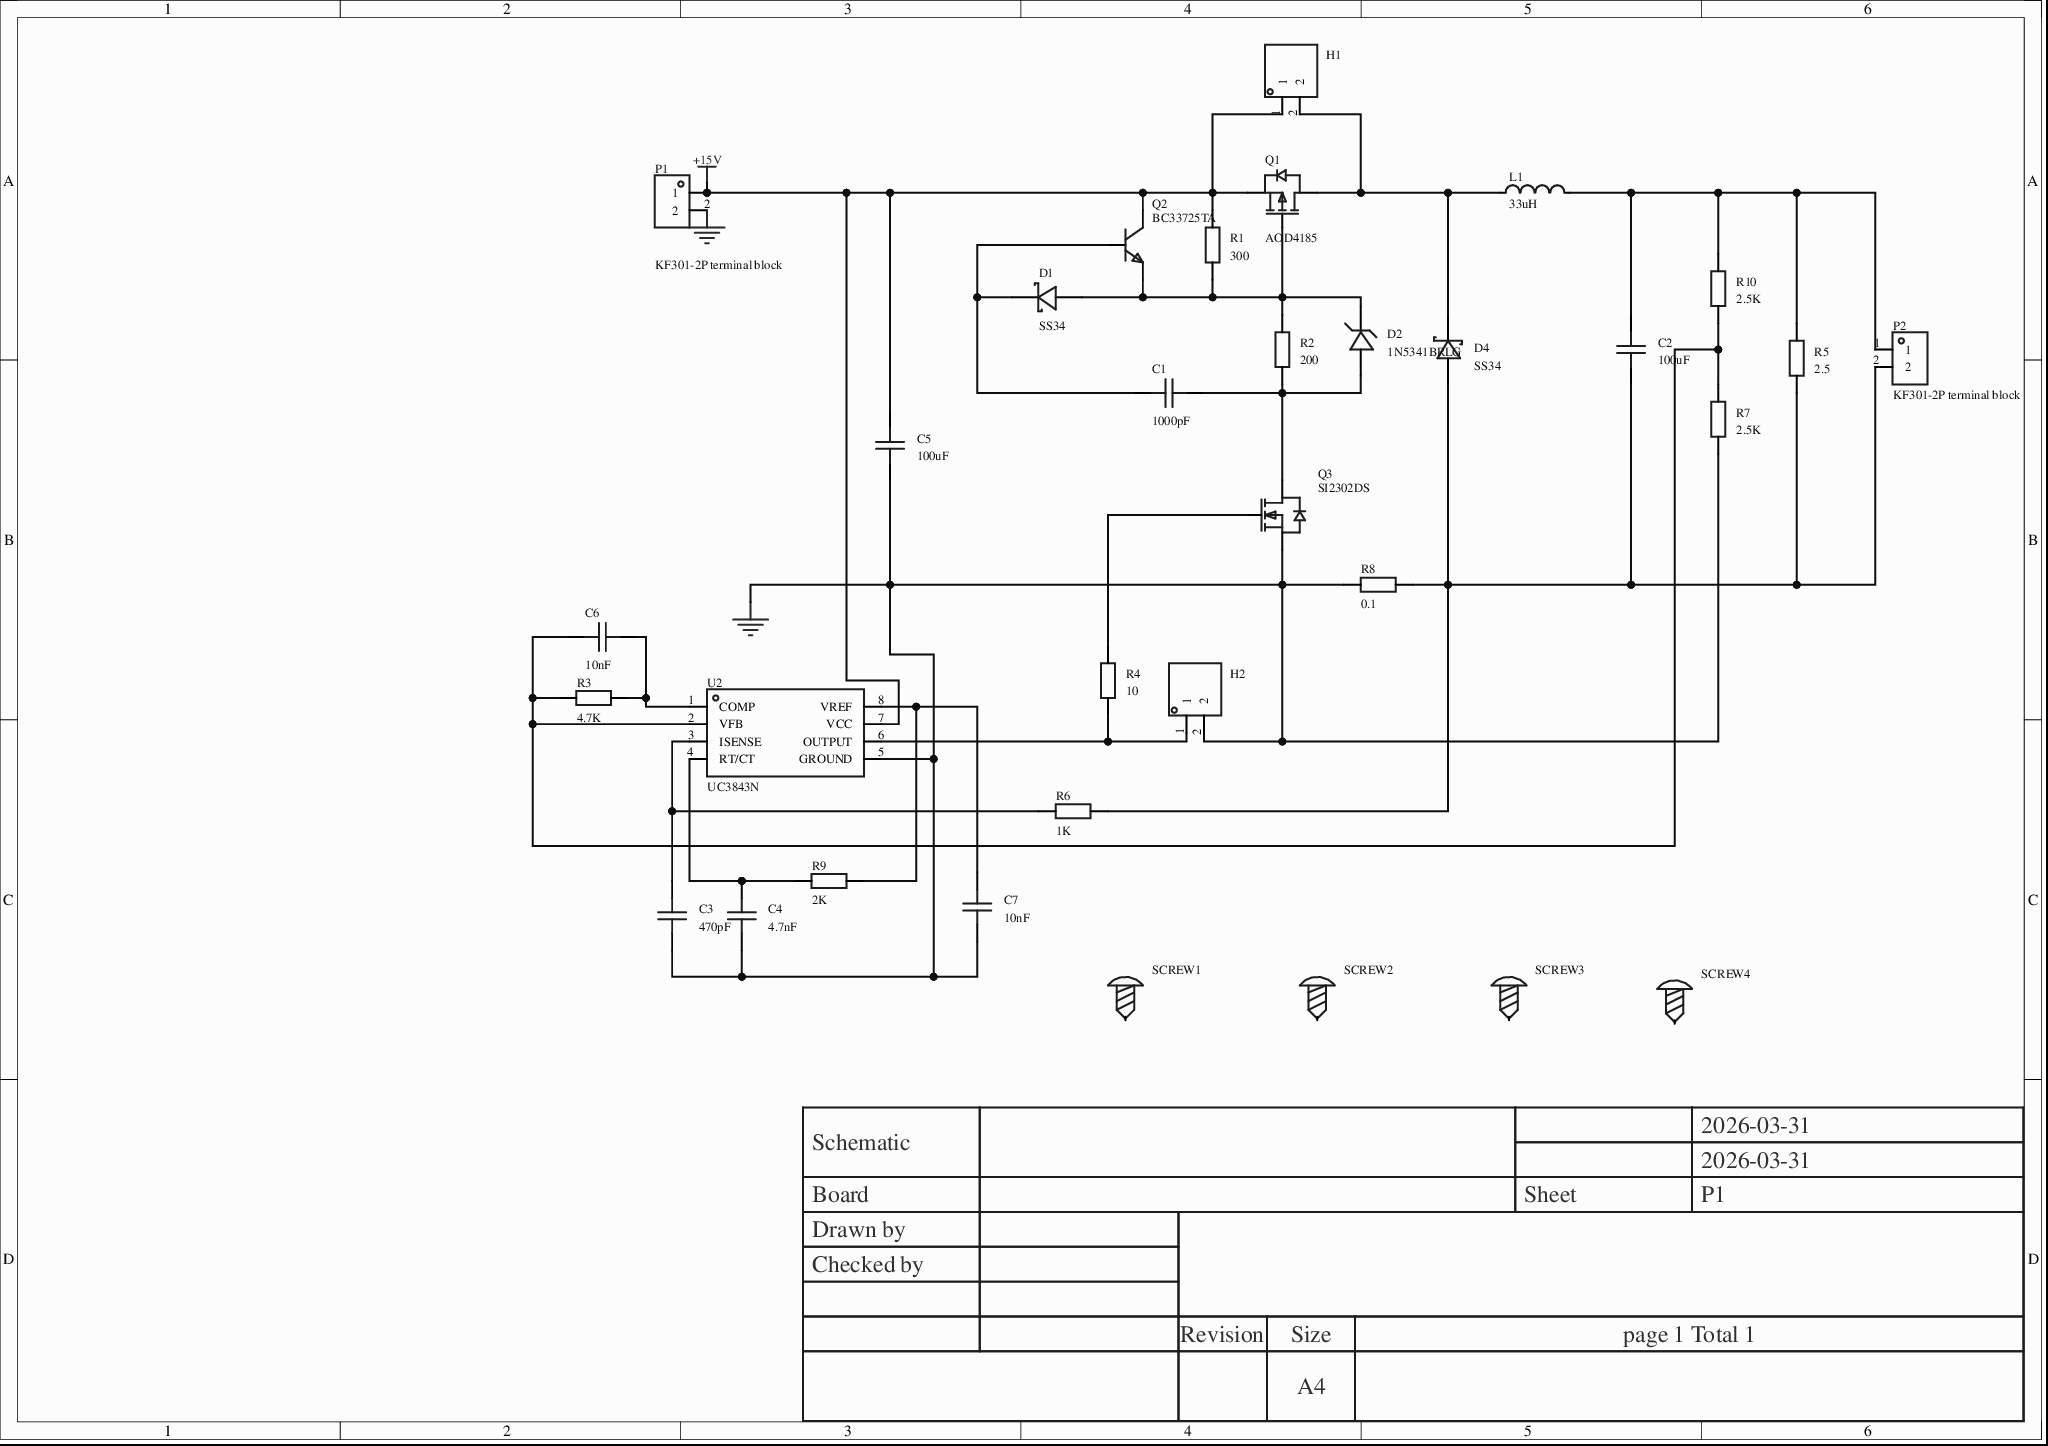
[diagram p0: MISC50807-3.schdoc]
# Altium project MISC50807-2.PrjPcb
1 sheet, 33 parts. Net scope: global (net labels, ports and power ports of the same name join across sheets).
Board file: MISC50807.pcbdoc

## Sheet MISC50807-3.schdoc
size 297 x 209 mm; Version: V1.0; @Project Name: MISC50807; @Update Date: 2026-04-21; @Create Date: 2026-04-21; @Board Name: MISC50807; @Create Time: 11:05:11; @Page Count: 1; @Page No: 1; @Schematic Name: MISC50807; @Update Time: 11:05:11; Size: A4

### Parts
C1  1000pF  [CAP-TH_L5.0-W2.5-P5.00-D1.0]
C2  100uF  [CAP-TH_BD8.0-P3.50-D0.6-FD_1]
C3  470pF  [CAP-TH_L5.0-W2.5-P5.00-D1.0]
C4  4.7nF  [CAP-TH_L5.0-W2.5-P5.00-D1.0]
C5  100uF  [CAP-TH_BD8.0-P3.50-D0.6-FD_1]
C6  10nF  [CAP-TH_L5.0-W2.5-P5.00-D1.0]
C7  10nF  [C0603]
D1  SS34  [DO-15_BD3.1-L6.7-P10.70-D0.8-RD]
D2  1N5341BRLG  [DO-15_BD3.1-L6.7-P10.70-D0.8-RD]
D4  SS34  [DO-15_BD3.1-L6.7-P10.70-D0.8-RD]
H1  (no value)  [HDR-TH_2P-P2.54-V-M-1]
H2  (no value)  [HDR-TH_2P-P2.54-V-M-1]
L1  33uH  [IND-TH_BD7.8-P5.00-D0.7]
P1  KF301-2P terminal block  [CONN-TH_XY301V-A-5.0-2P]
P2  KF301-2P terminal block  [CONN-TH_XY301V-A-5.0-2P]
Q1  AOD4185  [SOT-23-3_L2.9-W1.3-P1.90-LS2.4-L]
Q2  BC33725TA  [TO-92-3_L4.9-W3.7-P2.54-L]
Q3  SI2302DS  [SOT-23-3_L2.9-W1.3-P1.90-LS2.4-L]
R1  300  [Res_1/4W]
R2  200  [Res_1/4W]
R3  4.7K  [Res_1/4W]
R4  10  [Res_1/4W]
R5  2.5  [Res_1/4W]
R6  1K  [Res_1/4W]
R7  2.5K  [Res_1/4W]
R8  0.1  [Res_1/4W]
R9  2K  [Res_1/4W]
R10  2.5K  [Res_1/4W]
SCREW1  (no value)  [M3螺丝]
SCREW2  (no value)  [M3螺丝]
SCREW3  (no value)  [M3螺丝]
SCREW4  (no value)  [M3螺丝]
U2  UC3843N  [SOP-8_L5.1-W3.9-P1.27-LS6.0-BL]

### Nets
+15V: C5.2 H1.1 P1.1 Q1.3(S) Q2.1(C) R1.1 U2.7(VCC)
GND: C3.1 C4.1 C5.1 C7.1 H2.2 P1.2 Q3.2(S) R7.1 R8.1 U2.5(GROUND)
NetC1_1: C1.1 D1.1(C) Q2.2(B)
NetC1_2: C1.2 D2.2(A) Q3.3(D) R2.2
NetC2_1: C2.1 D4.2(A) P2.2 R5.1 R6.2 R8.2
NetC2_2: C2.2 L1.2 P2.1 R5.2 R10.2
NetC3_2: C3.2 R6.1 U2.3(ISENSE)
NetC4_2: C4.2 R9.1 U2.4(RT/CT)
NetC6_1: C6.1 R3.1 R7.2 R10.1 U2.2(VFB)
NetC6_2: C6.2 R3.2 U2.1(COMP)
NetC7_2: C7.2 R9.2 U2.8(VREF)
NetD1_2: D1.2(A) D2.1(C) Q1.1(G) Q2.3(E) R1.2 R2.1
NetD4_1: D4.1(C) H1.2 L1.1 Q1.2(D)
NetH2_1: H2.1 R4.2 U2.6(OUTPUT)
NetQ3_1: Q3.1(G) R4.1

Not connected (* = marked no-connect by the designer): SCREW1 1; SCREW2 1; SCREW3 1; SCREW4 1

### Notes on the sheet
- 2026-03-31
- Schematic
- Board
- Sheet
- P1
- Drawn by
- Checked by
- Revision
- Size
- A4
- page 1 Total 1

### Library data of the parts
C1-C4 = CAP_0603: Symbol: Capacitance; ConvertToPcb: yes; ModelId: ac125912035d415993ca9572d50418b10819f05c4eef4c71ace90d822a990e87; ModelName: C0603_L1.6-W0.8-H0.8; ModelTransform: 62.992,31.496,0,0,0,0,0,0,0; Device: CAP_0603; AddInBom: yes; Supplier Footprint: 0603
  C1: Value: 1000pF; FootprintName: CAP-TH_L5.0-W2.5-P5.00-D1.0
  C2: Value: 100uF; FootprintName: CAP-TH_BD8.0-P3.50-D0.6-FD_1
  C3: Value: 470pF; FootprintName: CAP-TH_L5.0-W2.5-P5.00-D1.0
  C4: Value: 4.7nF; FootprintName: CAP-TH_L5.0-W2.5-P5.00-D1.0
C5 C6 = CAP_0603: Symbol: Capacitance; 3D Model: ac125912035d415993ca9572d50418b10819f05c4eef4c71ace90d822a990e87; 3D Model Transform: 62.992,31.496,0,0,0,0,0,0,0; ConvertToPcb: yes; ModelName: C0603_L1.6-W0.8-H0.8; Device: CAP_0603; Supplier Footprint: 0603; AddInBom: yes
  C5: Value: 100uF; FootprintName: CAP-TH_BD8.0-P3.50-D0.6-FD_1
  C6: Value: 10nF; FootprintName: CAP-TH_L5.0-W2.5-P5.00-D1.0
C7 = CAP_0603: Symbol: CapAcitance; ConvertToPcb: yes; ModelId: ac125912035d415993ca9572d50418b10819f05c4eef4c71ace90d822a990e87; ModelName: C0603_L1.6-W0.8-H0.8; ModelTransform: 62.992,31.496,0,0,0,0,0,0,0; Device: CAP_0603; Value: 10nF; AddInBom: yes; Supplier Footprint: 0603; FootprintName: C0603
D1 D4 = SS34_C154551: Forward voltage (Vf): 500mV@3A; DC reverse voltage (Vr): 40V; Rectified current: 3A;; Manufacturer: onsemi(安森美); AddInBom: yes; Reverse Leakage Current (Ir): 500uA@40V; Operating Junction Temperature Range: -55℃~+150℃; Non-Repetitive Peak Forward Surge Current: 100A; ModelId: 181deed3e51b4528a83dd624c23bafda0819f05c4eef4c71ace90d822a990e87; ModelName: SMC_L6.9-W5.9-LS7.9-RD; ModelTransform: 314.96,236.22,0,0,0,0,0,0,0; Device: SS34_C154551; Symbol: SS34_C154551; FootprintName: DO-15_BD3.1-L6.7-P10.70-D0.8-RD; LCSC Part Name: 电压:40V 电流:3A; SupplierPart: C154551; ManufacturerPart: SS34; Supplier Footprint: SMC(DO-214AB); JLCPCB Part Class: Extended Part; Datasheet: https://example.com/datasheet/SS34/165893.html; Supplier: LCSC; ConvertToPcb: yes; Voltage - Forward(Vf@If): 500mV@3A; Voltage - DC Reverse(Vr): 40V; Current - Rectified: 3A
D2 = 1N5341BRLG: Diode configuration: standalone; Zener voltage (nominal): 6.2V; Zener voltage (range): 5.89V~6.51V; Tolerance: ±5%; Power: 5W; Reverse current (Ir): 1uA@3V; Impedance (Zzt): 1Ω;; Manufacturer: onsemi(安森美); AddInBom: yes; ModelId: ac7174ae5660404daaf53aba56e542fa0819f05c4eef4c71ace90d822a990e87; ModelName: DO-27_BD3.5-L8.6-P12.60-D1.3-RD; ModelTransform: 551.18,137.73354,0,0,0,0,0,0,-196.85; Device: 1N5341BRLG; Symbol: 1N5341BRLG; FootprintName: DO-15_BD3.1-L6.7-P10.70-D0.8-RD; LCSC Part Name: 6.2V ±5% 5W; SupplierPart: C9707; ManufacturerPart: 1N5341BRLG; Supplier Footprint: AXIAL LEAD; JLCPCB Part Class: Extended Part; Datasheet: https://example.com/upload/public/pdf/source/20121103/1457706546069.pdf; Supplier: LCSC; ConvertToPcb: yes; Diode Configuration: Standalone; Zener Voltage (Nom): 6.2V; Zener Voltage (Range): 5.89V~6.51V; Power Dissipation: 5W; Reverse Leakage Current (Ir): 1uA@3V; Zener Impedance (Zzt): 1Ω
H1 H2 = HDR-M_2.54_1x2P: Symbol: 210S-1*2P L=11.6MMGold-plated black; ConvertToPcb: yes; ModelId: 79b2e9f2d70a4d68a1b7098f27c6d4c50819f05c4eef4c71ace90d822a990e87; ModelName: HDR-M-2.54_1x2; ModelTransform: 200,100,0,0,0,0,0,0,-118.11; Device: HDR-M_2.54_1x2P; FootprintName: HDR-TH_2P-P2.54-V-M-1; AddInBom: yes; SupplierPart: C124375; Supplier Footprint: 插件
L1 = L_0603: Symbol: SDFL1608S100KTF; AddInBom: yes; ModelId: 2bc5ec593d464d6ba9807aec0b5673c20819f05c4eef4c71ace90d822a990e87; ModelName: L0603_L1.6-W0.8-H0.5_BEAD; ModelTransform: 62.992,31.496,0,180,0,0,0.094,0.629,0; Device: L_0603; Value: 33uH; FootprintName: IND-TH_BD7.8-P5.00-D0.7; Supplier Footprint: L0603; ConvertToPcb: yes
P1 P2 = KF301-2P接线端子: AddInBom: yes; ModelId: ef7ead88b0f2448d904975b26718870f0819f05c4eef4c71ace90d822a990e87; ModelTransform: 417.322,299.212,0,0,0,0,11.811,-7.835,-157.48; Device: KF301-2P terminal block; Symbol: KF301-2P terminal block; FootprintName: CONN-TH_XY301V-A-5.0-2P; LCSC Part Name: KF301-2P接线端子; SupplierPart: C9900016950; ManufacturerPart: KF301-2P接线端子; Supplier Footprint: CK301-2P; JLCPCB Part Class: Extended Part; Supplier: LCSC; ConvertToPcb: yes; ModelName: CONN-TH_XY301V-A-5.0-2P
Q1 = AOD4185_C400894: Type: 1 P-channel; Drain-source voltage (Vdss): 40V; Continuous drain current (Id): 40A; On-resistance (RDS(on)@Vgs,Id): 20mΩ@4.5V,15A; Power (Pd): 62.5W; Threshold voltage (Vgs(th)@Id): 1.7V@250uA;; Manufacturer: AOS; AddInBom: yes; Total Gate Charge (Qg@Vgs): 42nC@10V; Input Capacitance (Ciss@Vds): 2.55nF@20V; Reverse Transfer Capacitance (Crss@Vds): 190pF@20V; ModelId: dee852f3c6b348a2b9d5be5dd32440810819f05c4eef4c71ace90d822a990e87; ModelName: TO-252-3_L6.6-W6.1-P4.57-LS9.9-BR-CW; ModelTransform: 258.97184,390.1567,0,90,0,0,-35.433,0,0; Device: AOD4185_C400894; Symbol: AOD4185_C400894; FootprintName: SOT-23-3_L2.9-W1.3-P1.90-LS2.4-L; LCSC Part Name: 1个P沟道 耐压:40V 电流:40A; SupplierPart: C400894; ManufacturerPart: AOD4185; Supplier Footprint: TO-252(DPAK); JLCPCB Part Class: Extended Part; Datasheet: https://example.com/upload/public/pdf/source/20190627/C400894_921958B6CB7B7C674397E60AAED89785.pdf; Supplier: LCSC; ConvertToPcb: yes; Drain Source Voltage (Vdss): 40V; Continuous Drain Current (Id): 40A; Drain Source On Resistance (RDS(on)@Vgs,Id): 20mΩ@4.5V,15A; Power Dissipation (Pd): 62.5W; Gate Threshold Voltage (Vgs(th)@Id): 1.7V@250uA; Operating Temperature: -55℃~+175℃
Q2 = BC33725TA: Transistor type: NPN; Collector current (Ic): 800mA; Collector-emitter breakdown voltage (Vceo): 45V; Power dissipation (Pd): 625mW; DC current gain (hFE): 100@100mA,1V;; Manufacturer: onsemi(安森美); AddInBom: yes; Transition frequency(fT): 100MHz; Current - Collector Cutoff: 100nA; Vce Saturation(VCE(sat)): 700mV@500mA,50mA; Emitter-Base Voltage(Vebo): 5V; Number: 1 NPN; ModelId: ff77d7980f5c4c0980cec2e309db67c40819f05c4eef4c71ace90d822a990e87; ModelTransform: 222.047,139.764,0,180,0,0,0,28.661,-196.85; Device: BC33725TA; Symbol: BC33725TA; FootprintName: TO-92-3_L4.9-W3.7-P2.54-L; LCSC Part Name: NPN 电流:800mA 电压:45V; SupplierPart: C236942; ManufacturerPart: BC33725TA; Supplier Footprint: TO-92-3; JLCPCB Part Class: Extended Part; Datasheet: https://example.com/datasheet/BC33725TA/236369.html; Supplier: LCSC; ConvertToPcb: yes; type: NPN; Current - Collector(Ic): 800mA; Collector - Emitter Voltage VCEO: 45V; Pd - Power Dissipation: 625mW; DC Current Gain: 100@100mA,1V; Operating Temperature: -55℃~+150℃; ModelName: TO-92-3_L4.9-W3.7-P2.54-L
Q3 = SI2302DS: Quantity: 1 N-channel; Drain-source voltage (Vdss): 20V; Continuous drain current (Id): 2.8A; On-resistance (RDS(on)): 120mΩ@2.5V; 83mΩ@4.5V; Power dissipation (Pd): 900mW; Threshold voltage (Vgs(th)): 1.5V;; Manufacturer: TECH PUBLIC(台舟); AddInBom: yes; Input Capacitance(Ciss): 880pF; Output Capacitance(Coss): 270pF; ModelId: c62791f0466c4ae2a892c056b845b0ca0819f05c4eef4c71ace90d822a990e87; ModelName: SOT-23-3P_L2.9-W1.3-H1.0-LS2.4-P0.95; ModelTransform: 98.425,114.173,0,180,0,0,0.0005,-0.0005,0; Device: SI2302DS; Symbol: SI2302DS; FootprintName: SOT-23-3_L2.9-W1.3-P1.90-LS2.4-L; LCSC Part Name: N沟道增强型场效应晶体管; SupplierPart: C5310967; ManufacturerPart: SI2302DS; Supplier Footprint: SOT-23; JLCPCB Part Class: Extended Part; Datasheet: https://example.com/datasheet/SI2302DS/6066823.html; Supplier: LCSC; ConvertToPcb: yes; Number: 1 N-channel; Drain to Source Voltage: 20V; Current - Continuous Drain(Id): 2.8A; RDS(on): 120mΩ@2.5V; 83mΩ@4.5V; Pd - Power Dissipation: 900mW; Gate Threshold Voltage (Vgs(th)): 1.5V; Type: N-channel
R1-R3 R5-R10 = Res_0603: Symbol: Resistor; ConvertToPcb: yes; ModelId: fc143cca1e79419f9cd78b61e9279f080819f05c4eef4c71ace90d822a990e87; ModelName: R0603; ModelTransform: 31.8897,63.7794,0,90,0,0,0,0,0; Device: Res_0603; FootprintName: Res_1/4W; AddInBom: yes; Supplier Footprint: 0603
  R1: Value: 300
  R2: Value: 200
  R3: Value: 4.7K
  R5: Value: 2.5
  R6: Value: 1K
  R7 R10: Value: 2.5K
  R8: Value: 0.1
  R9: Value: 2K
R4 = Res_0603: Symbol: Resistor; 3D Model: fc143cca1e79419f9cd78b61e9279f080819f05c4eef4c71ace90d822a990e87; 3D Model Transform: 31.8897,63.7794,0,90,0,0,0,0,0; ConvertToPcb: yes; ModelName: R0603; Device: Res_0603; Value: 10; Supplier Footprint: 0603; FootprintName: Res_1/4W; AddInBom: yes
SCREW1-SCREW4 = M3螺丝: Device: M3 screw; Symbol: Screw hole; ConvertToPcb: yes; FootprintName: M3 screw; AddInBom: yes; Supplier Footprint: 插件
U2 = UC3843N: Operating voltage: 12V~28V;; Manufacturer: TI(德州仪器); Symbol: UC3843N_C1530280; AddInBom: yes; ModelId: 28221afe73f64733a5f69edf09cc82000819f05c4eef4c71ace90d822a990e87; ModelName: PDIP-8_L9.3-W6.4-P2.54-LS7.9-BL-1; ModelTransform: 366.141,322.834,0,0,0,0,0,0,-118.11; Device: UC3843N; FootprintName: SOP-8_L5.1-W3.9-P1.27-LS6.0-BL; LCSC Part Name: UC3843N; SupplierPart: C1530280; ManufacturerPart: UC3843N; Supplier Footprint: PDIP-8; JLCPCB Part Class: Extended Part; Supplier: LCSC; ConvertToPcb: yes; Voltage - Supply: 12V~28V; Operating Temperature: 0℃~+70℃@(TA)